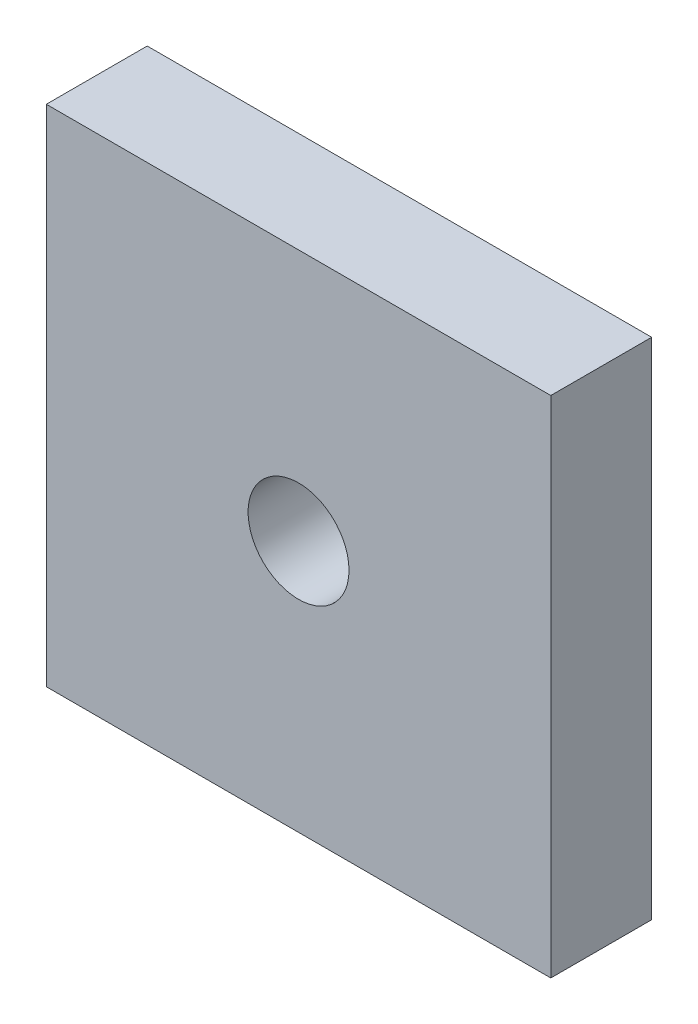
SolidWorks part; units mm, degrees
ref_plane "前视基准面" through (0, 0, 0) normal (0, 0, 1) x (1, 0, 0)
ref_plane "上视基准面" through (0, 0, 0) normal (0, 1, 0) x (1, 0, 0)
ref_plane "右视基准面" through (0, 0, 0) normal (1, 0, 0) x (0, 0, -1)
sketch "草图1" plane through (0, 0, 0) normal (0, 0, 1) x (1, 0, 0)
  line L0 (0, 0) -> (0, 50)
  line L1 (0, 50) -> (50, 50)
  line L2 (50, 50) -> (50, 0)
  line L3 (50, 0) -> (0, 0)
  circle A0 centre (25, 25) radius 5
extrude "凸台-拉伸1" add sketch "草图1" along normal blind 10
